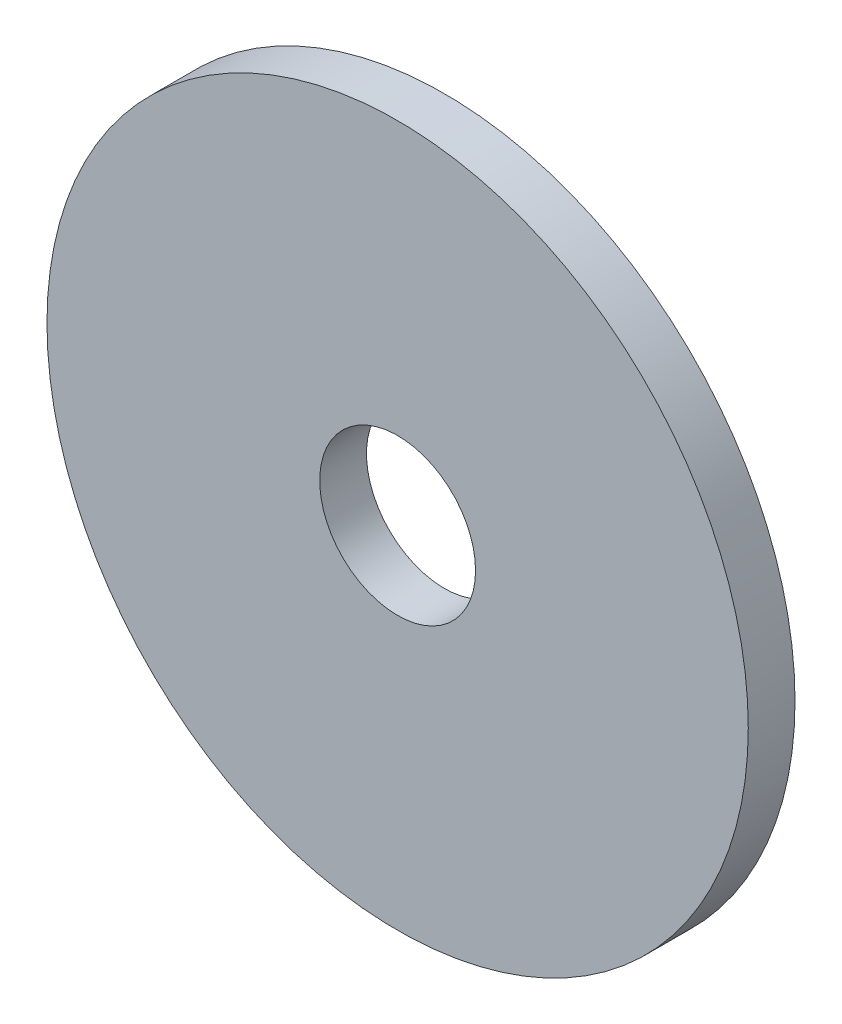
from build123d import *

# Parameters (mm, degrees)
SKETCH_1_R      = 22.5
SKETCH_1_R_2    = 5
EXTRUDE_1_DEPTH = 3


with BuildPart() as part:
    # 草图1 → 凸台-拉伸1 (new body)
    with BuildSketch(Plane.XY):
        Circle(SKETCH_1_R)
        Circle(SKETCH_1_R_2, mode=Mode.SUBTRACT)
    extrude(amount=EXTRUDE_1_DEPTH)


solid = part.part
